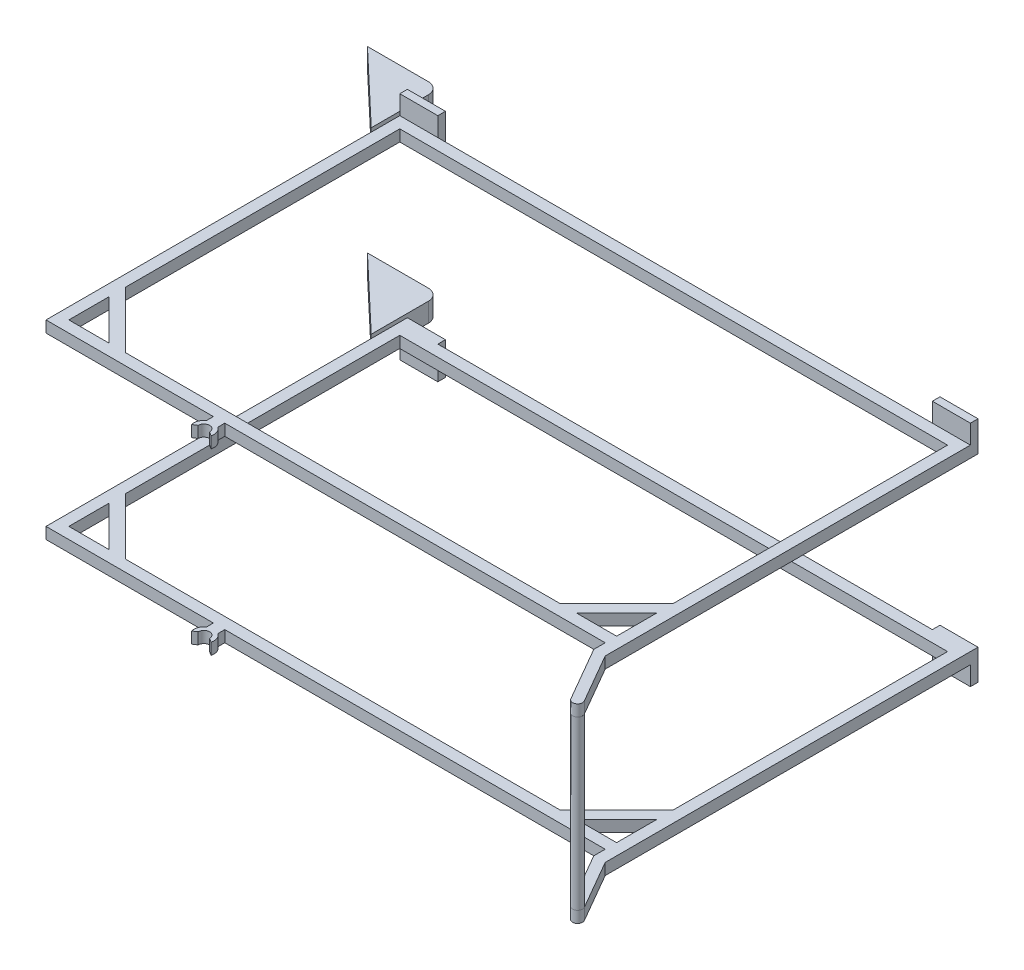
SolidWorks part; units mm, degrees
ref_plane "Front" through (0, 0, 0) normal (0, 0, 1) x (1, 0, 0)
ref_plane "Top" through (0, 0, 0) normal (0, 1, 0) x (1, 0, 0)
ref_plane "Right" through (0, 0, 0) normal (1, 0, 0) x (0, 0, -1)
sketch "Sketch1" plane through (0, 0, 0) normal (0, 0, 1) x (1, 0, 0)
  line L1 (0, 0) -> (-1500, 0)
  line L2 (0, 0) -> (0, -500)
  line L3 (0, -500) -> (-1500, -500)
  line L4 (-1500, 0) -> (-1500, -500)
  dimension "D1" = 500
  dimension "D2" = 1500
extrude "Boss-Extrude1" add sketch "Sketch1" along normal blind 30
sketch "Sketch2" plane through (0, 0, 30) normal (0, 0, 1) x (1, 0, 0)
  line L1 (-1500, -500) -> (-1470, -500)
  line L2 (-1500, -500) -> (-1500, -470)
  line L3 (-1500, -470) -> (-1470, -470)
  line L4 (-1470, -500) -> (-1470, -470)
  line L5 (-1500, 0) -> (-1470, 0)
  line L6 (-1500, 0) -> (-1500, -30)
  line L7 (-1500, -30) -> (-1470, -30)
  line L8 (-1470, 0) -> (-1470, -30)
  line L9 (0, 0) -> (-30, 0)
  line L10 (0, 0) -> (0, -30)
  line L11 (0, -30) -> (-30, -30)
  line L12 (-30, 0) -> (-30, -30)
  line L13 (0, -500) -> (-30, -500)
  line L14 (0, -500) -> (0, -470)
  line L15 (0, -470) -> (-30, -470)
  line L16 (-30, -500) -> (-30, -470)
  dimension "D1" = 30
  dimension "D2" = 30
  dimension "D3" = 30
  dimension "D4" = 30
  dimension "D5" = 30
  dimension "D6" = 30
extrude "Boss-Extrude2" add sketch "Sketch2" along normal blind 900
sketch "Sketch3" plane through (0, -500, 0) normal (0, -1, 0) x (1, 0, 0)
  line L0 (0, 930) -> (0, 0) construction
  line L1 (-1500, 930) -> (0, 930)
  line L2 (-1500, 930) -> (-1500, 900)
  line L3 (-1500, 900) -> (-1363.934, 900)
  line L4 (0, 930) -> (0, 900)
  line L5 (-1363.934, 900) -> (-1470, 793.934)
  line L6 (-1470, 930) -> (-1470, 30) construction
  line L7 (-1321.5076, 900) -> (-1470, 751.5076)
  line L8 (-1470, 793.934) -> (-1470, 751.5076)
  line L9 (-1321.5076, 900) -> (-178.4924, 900)
  line L10 (-750, 930) -> (-750, 448.9742) construction
  line L11 (-178.4924, 900) -> (-30, 751.5076)
  line L12 (-136.066, 900) -> (-30, 793.934)
  line L13 (-136.066, 900) -> (0, 900)
  line L14 (-30, 793.934) -> (-30, 751.5076)
  dimension "D1" = 30
  dimension "D2" = 45
  dimension "D3" = 150
  dimension "D4" = 30
extrude "Boss-Extrude3" add sketch "Sketch3" against normal blind 30
ref_plane "Plane1" through (0, -250, 0) normal (0, 1, 0) x (1, 0, 0)
mirror "Mirror2" about plane through (0, -250, 0) normal (0, 1, 0) of "Boss-Extrude3"
sketch "Sketch4" plane through (0, 0, 930) normal (0, 0, 1) x (1, 0, 0)
  line L0 (0, 0) -> (-1500, 0) construction
  line L1 (0, -500) -> (-30, -500)
  line L2 (0, -500) -> (0, 0)
  line L3 (0, 0) -> (-30, 0)
  line L4 (-30, -500) -> (-30, 0)
  dimension "D1" = 30
extrude "Boss-Extrude4" add sketch "Sketch4" along normal blind 30
sketch "Sketch5" plane through (0, -500, 0) normal (0, -1, 0) x (1, 0, 0)
  line L0 (0, 960) -> (75, 1089.9038)
  line L1 (30.2363, 1064.3324) -> (37.5, 1076.9134)
  line L2 (37.5, 1076.9134) -> (52.5, 1102.8942)
  line L5 (-30, 960) -> (0, 960)
  line L6 (-30, 960) -> (30.2363, 1064.3324)
  arc A2 (52.5, 1102.8942) -> (75, 1089.9038) centre (63.6593, 1096.2418) cw
  dimension "D3" = 150
extrude "Boss-Extrude5" add sketch "Sketch5" against normal blind 30
mirror "Mirror3" about plane through (0, -250, 0) normal (0, 1, 0) of "Boss-Extrude5"
sketch "Sketch6" plane through (0, -500, 0) normal (0, -1, 0) x (1, 0, 0)
  circle A1 centre (63.6593, 1096.2418) radius 12.9904
  arc A2 (75, 1089.9038) -> (52.5, 1102.8942) centre (63.6593, 1096.2418) ccw construction
extrude "Boss-Extrude6" add sketch "Sketch6" against normal up to surface (500 mm away) up to face at (-365.7619, 0, 747.9865)
sketch "Sketch8" plane through (0, -500, 0) normal (0, -1, 0) x (1, 0, 0)
  line L16 (-1500, 930) -> (-30, 930) construction
  line L17 (-1060, 930) -> (-1030, 930)
  line L21 (-1060, 930) -> (-1060, 948.1349)
  line L25 (-1060.0607, 970.038) -> (-1070.6617, 976.6756)
  line L26 (-1029.9393, 970.038) -> (-1019.3383, 976.6756)
  line L27 (-30, 751.5076) -> (-30, 30) construction
  line L28 (-1030, 948.1349) -> (-1030, 930)
  arc A13 (-1070.6617, 976.6756) -> (-1060, 948.1349) centre (-1045, 970) ccw
  arc A14 (-1060.0607, 970.038) -> (-1029.9393, 970.038) centre (-1045, 970) ccw
  arc A16 (-1030, 948.1349) -> (-1019.3383, 976.6756) centre (-1045, 970) ccw
  dimension "D2" = 1000
  dimension "D1" = 30
extrude "Boss-Extrude7" add sketch "Sketch8" against normal blind 30
mirror "Mirror4" about plane through (0, -250, 0) normal (0, 1, 0) of "Boss-Extrude7"
sketch "Sketch10" plane through (0, -500, 0) normal (0, -1, 0) x (1, 0, 0)
  line L1 (-1500, 75) -> (-1500, -105)
  line L2 (-1500, 930) -> (-1500, 0) construction
  line L3 (-1500, -105) -> (-1690, -105)
  line L4 (-1500, 75) -> (-1690, -105)
  line L5 (-1500, 0) -> (0, 0) construction
  dimension "D1" = 180
  dimension "D2" = 190
  dimension "D3" = 75
extrude "Boss-Extrude8" add sketch "Sketch10" against normal blind 300
fillet "Fillet1" radius 30 1 edges at (-1500, -350, -105)
sketch "Sketch11" plane through (0, 0, 0) normal (1, 0, 0) x (0, 0, -1)
  line L1 (-960, -500) -> (0, -500)
  line L2 (-960, -500) -> (-960, 0)
  line L3 (-960, 0) -> (0, 0)
  line L4 (0, -500) -> (0, 0)
extrude "Boss-Extrude9" add sketch "Sketch11" against normal up to surface (30 mm away) up to face at (-30, -15, 390.7538)
sketch "Sketch12" plane through (0, 0, 0) normal (1, 0, 0) x (0, 0, -1)
  line L1 (-50, -460) -> (-90, -460)
  line L2 (-50, -460) -> (-50, -240)
  line L3 (-50, -240) -> (-90, -240)
  line L4 (-90, -460) -> (-90, -240)
  line L5 (0, -500) -> (0, 0) construction
  line L8 (-960, -500) -> (0, -500) construction
  dimension "D1" = 50
  dimension "D2" = 220
  dimension "D3" = 40
  dimension "D4" = 40
extrude "Cut-Extrude1" cut sketch "Sketch12" against normal blind 300
sketch "Sketch13" plane through (0, 0, 0) normal (1, 0, 0) x (0, 0, -1)
  line L1 (-960, -470) -> (193.0012, -470)
  line L2 (-960, -470) -> (-960, -30)
  line L3 (-960, -30) -> (193.0012, -30)
  line L4 (193.0012, -470) -> (193.0012, -30)
extrude "Cut-Extrude2" cut sketch "Sketch13" against normal through all
ref_plane "Plane2" through (0, -485, 0) normal (0, -1, 0) x (-1, 0, 0)
sketch "Sketch15" plane through (0, -485, 0) normal (0, -1, 0) x (-1, 0, 0)
  line L0 (1500, -75) -> (1500, 0)
  line L10 (-52.5, -1102.8942) -> (30, -960)
  line L11 (30, -960) -> (30, -930)
  line L12 (1030, -930) -> (1030, -948.1349)
  line L13 (1030, -930) -> (1030, -948.1349)
  line L17 (30, -930) -> (1030, -930)
  line L21 (1019.3383, -976.6756) -> (1029.9393, -970.038)
  line L22 (1019.3383, -976.6756) -> (1029.9393, -970.038)
  line L23 (1500, -930) -> (1500, -75)
  line L24 (1500, -75) -> (1690, 105)
  line L25 (1690, 105) -> (1530, 105)
  line L26 (1500, 75) -> (1500, 0)
  line L27 (1500, 0) -> (0, 0)
  line L28 (0, 0) -> (0, -960)
  line L29 (1060, -930) -> (1500, -930)
  line L39 (1500, -75) -> (1690, 105)
  line L40 (1690, 105) -> (1530, 105)
  line L41 (1500, 75) -> (1500, 0)
  line L42 (0, -960) -> (-75, -1089.9038)
  line L43 (1060.0607, -970.038) -> (1070.6617, -976.6756)
  line L44 (1060.0607, -970.038) -> (1070.6617, -976.6756)
  line L45 (1060, -948.1349) -> (1060, -930)
  line L46 (1060, -948.1349) -> (1060, -930)
  arc A5 (1030, -948.1349) -> (1019.3383, -976.6756) centre (1045, -970) ccw
  arc A6 (1030, -948.1349) -> (1019.3383, -976.6756) centre (1045, -970) ccw
  arc A7 (1060.0607, -970.038) -> (1029.9393, -970.038) centre (1045, -970) ccw
  arc A8 (1530, 105) -> (1500, 75) centre (1530, 75) ccw
  arc A9 (1060.0607, -970.038) -> (1029.9393, -970.038) centre (1045, -970) ccw
  arc A13 (1530, 105) -> (1500, 75) centre (1530, 75) ccw
  arc A14 (1070.6617, -976.6756) -> (1060, -948.1349) centre (1045, -970) ccw
  arc A15 (1070.6617, -976.6756) -> (1060, -948.1349) centre (1045, -970) ccw
  arc A16 (-75, -1089.9038) -> (-52.5, -1102.8942) centre (-63.6593, -1096.2418) ccw
  arc A17 (-75, -1089.9038) -> (-52.5, -1102.8942) centre (-63.6593, -1096.2418) ccw
  dimension "D1" = 0
extrude "Boss-Extrude11" add sketch "Sketch15" along normal mid plane 50 contours L41 L0 L39 L40 A13
mirror "Mirror5" about plane through (0, -250, 0) normal (0, 1, 0) of "Boss-Extrude11"
sketch "Sketch16" plane through (0, 0, 0) normal (0, 0, -1) x (-1, 0, 0)
  line L1 (1500, -30) -> (1400, -30)
  line L2 (1500, -30) -> (1500, 50)
  line L3 (1500, 50) -> (1400, 50)
  line L4 (1400, -30) -> (1400, 50)
  line L5 (1500, -470) -> (1400, -470)
  line L6 (1500, -470) -> (1500, -555.9409)
  line L7 (1500, -555.9409) -> (1400, -555.9409)
  line L8 (1400, -470) -> (1400, -555.9409)
  line L9 (0, -470) -> (100, -470)
  line L10 (0, -470) -> (0, -550)
  line L11 (0, -550) -> (100, -550)
  line L12 (100, -470) -> (100, -550)
  line L13 (0, -30) -> (100, -30)
  line L14 (0, -30) -> (0, 50)
  line L15 (0, 50) -> (100, 50)
  line L16 (100, -30) -> (100, 50)
  dimension "D1" = 100
  dimension "D2" = 80
  dimension "D3" = 80
  dimension "D4" = 100
  dimension "D5" = 100
  dimension "D6" = 80
  dimension "D7" = 100
extrude "Boss-Extrude12" add sketch "Sketch16" along normal blind 20
